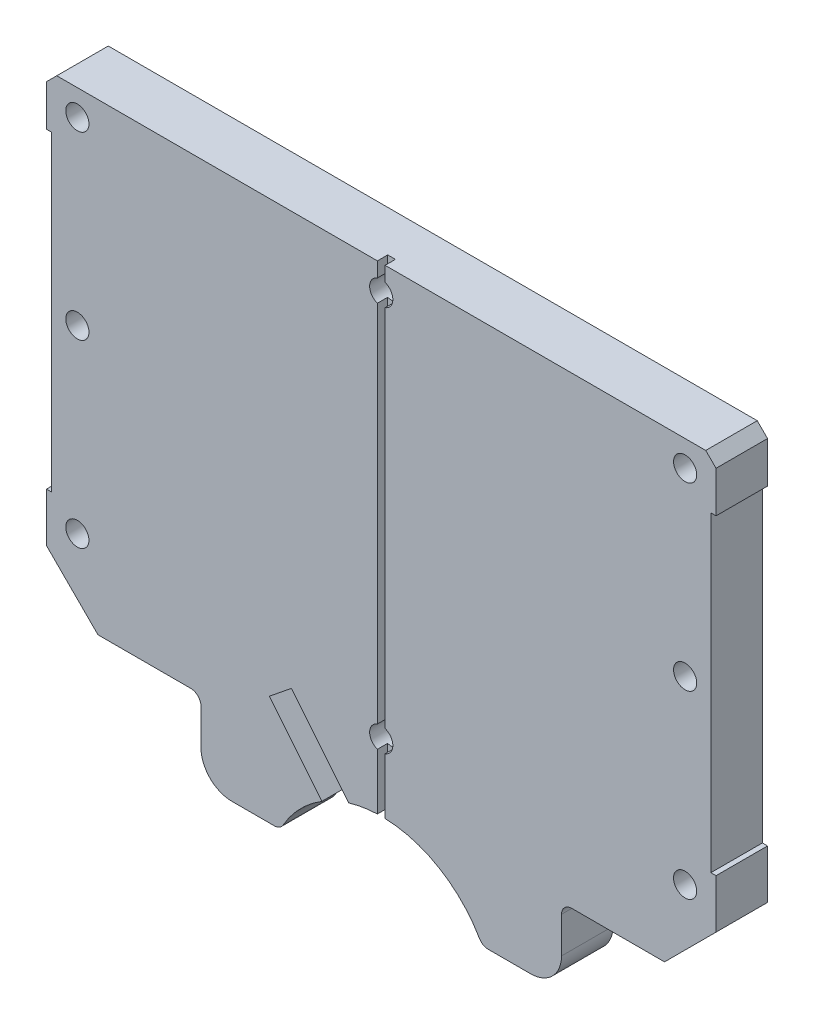
from build123d import *

# Parameters (mm, degrees)
SKETCH1_W                                            = 130
SKETCH1_H                                            = 105
BOSS_EXTRUDE1_DEPTH                                  = 5
SKETCH3_R                                            = 22
CUT_EXTRUDE2_DEPTH                                   = 85.150163399
SKETCH7_W                                            = 30
SKETCH7_H                                            = 10
CUT_EXTRUDE5_DEPTH                                   = 15
FILLET1_R                                            = 6
CHAMFER1_SIZE                                        = 10
FILLET2_R                                            = 2
CUT_EXTRUDE8_DEPTH                                   = 85.150163399
FILLET3_R                                            = 2
CHAMFER2_SIZE                                        = 2
SKETCH15_W                                           = 1
SKETCH15_H                                           = 60.5
CUT_EXTRUDE10_DEPTH                                  = 85.150163399
HOLE_SIZE_PER_SOCKET_HEAD_CAP_SCREW_TYPE_D           = 4.5
HOLE_SIZE_PER_SOCKET_HEAD_CAP_SCREW_TYPE_CBORE_D     = 8
HOLE_SIZE_PER_SOCKET_HEAD_CAP_SCREW_TYPE_CBORE_DEPTH = 4.5
M3_TAPPED_HOLE1_D                                    = 2.5
M3_TAPPED_HOLE1_DEPTH                                = 8.5
M3_TAPPED_HOLE1_TIP                                  = 0.751075774
SKETCH20_W                                           = 1.5
SKETCH20_H                                           = 105
CUT_EXTRUDE11_DEPTH                                  = 2


with BuildPart() as part:
    # Sketch1 → Boss-Extrude1 (new, symmetric)
    with BuildSketch(Plane.XY):
        Rectangle(SKETCH1_W, SKETCH1_H)
    extrude(amount=BOSS_EXTRUDE1_DEPTH, both=True)

    # Sketch3 → Cut-Extrude2 (cut, through all)
    with BuildSketch(Plane.XY.offset(5)):
        with Locations((0, -62.5)):
            Circle(SKETCH3_R)
    extrude(amount=-CUT_EXTRUDE2_DEPTH, mode=Mode.SUBTRACT)

    # Sketch7 → Cut-Extrude5 (cut)
    with BuildSketch(Plane.XZ.offset(52.5)):
        with Locations((-50, 0)):
            Rectangle(SKETCH7_W, SKETCH7_H)
        with Locations((50, 0)):
            Rectangle(SKETCH7_W, SKETCH7_H)
    extrude(amount=-CUT_EXTRUDE5_DEPTH, mode=Mode.SUBTRACT)

    # Fillet1
    fillet1_edges = [part.edges().sort_by_distance(p)[0] for p in [
        (-35, -52.5, 0),
        (35, -52.5, 0),
    ]]
    fillet(fillet1_edges, radius=FILLET1_R)

    # Chamfer1
    chamfer1_edges = [part.edges().sort_by_distance(p)[0] for p in [
        (-65, -37.5, 0),
        (65, -37.5, 0),
    ]]
    chamfer(chamfer1_edges, length=CHAMFER1_SIZE)

    # Fillet2
    fillet2_edges = [part.edges().sort_by_distance(p)[0] for p in [
        (-35, -37.5, 0),
        (35, -37.5, 0),
    ]]
    fillet(fillet2_edges, radius=FILLET2_R)

    # Sketch10 → Cut-Extrude8 (cut, through all)
    with BuildSketch(Plane.XY.offset(5)):
        Polygon((-21.710710609, -31.184123297), (-17.436407821, -27.722861146), (-4.85, -43.265780375), (-9.124302788, -46.727042526), align=None)
    extrude(amount=-CUT_EXTRUDE8_DEPTH, mode=Mode.SUBTRACT)

    # Fillet3
    fillet3_edges = [part.edges().sort_by_distance(p)[0] for p in [
        (-19.595917942, -52.5, 0),
        (19.595917942, -52.5, 0),
    ]]
    fillet(fillet3_edges, radius=FILLET3_R)

    # Chamfer2
    chamfer2_edges = [part.edges().sort_by_distance(p)[0] for p in [
        (-65, 52.5, 0),
        (65, 52.5, 0),
    ]]
    chamfer(chamfer2_edges, length=CHAMFER2_SIZE)

    # Sketch15 → Cut-Extrude10 (cut, through all)
    with BuildSketch(Plane(origin=(0, 0, -5), x_dir=(-1, 0, 0), z_dir=(0, 0, -1))):
        with Locations((-64.5, 12.25)):
            Rectangle(SKETCH15_W, SKETCH15_H)
        with Locations((64.5, 12.25)):
            Rectangle(SKETCH15_W, SKETCH15_H)
    extrude(amount=-CUT_EXTRUDE10_DEPTH, mode=Mode.SUBTRACT)

    # Hole size per socket head cap screw type 0 (through all)
    with Locations(Plane(origin=(-18.523886338, 13.049633662, -5), x_dir=(1, 0, 0), z_dir=(0, 0, -1))):
        with Locations((77.523886338, -34.450366338), (18.523886338, -34.450366338), (-40.476113662, -34.450366338), (-40.476113662, 0.549633662), (-40.476113662, 35.549633662), (18.523886338, 40.549633662), (77.523886338, 35.549633662), (77.523886338, 0.549633662)):
            CounterBoreHole(HOLE_SIZE_PER_SOCKET_HEAD_CAP_SCREW_TYPE_D / 2, HOLE_SIZE_PER_SOCKET_HEAD_CAP_SCREW_TYPE_CBORE_D / 2, HOLE_SIZE_PER_SOCKET_HEAD_CAP_SCREW_TYPE_CBORE_DEPTH)

    # M3 Tapped Hole1
    with Locations(Plane(origin=(-15.568631127, 3.135719595, -5), x_dir=(1, 0, 0), z_dir=(0, 0, -1))):
        with Locations((-7.431368873, 28.635719595)):
            Hole(M3_TAPPED_HOLE1_D / 2, depth=M3_TAPPED_HOLE1_DEPTH)
            with Locations((0, 0, -(M3_TAPPED_HOLE1_DEPTH + M3_TAPPED_HOLE1_TIP / 2))):  # 118° drill point
                Cone(0, M3_TAPPED_HOLE1_D / 2, M3_TAPPED_HOLE1_TIP, mode=Mode.SUBTRACT)

    # Sketch20 → Cut-Extrude11 (cut)
    with BuildSketch(Plane.XY.offset(5)):
        Rectangle(SKETCH20_W, SKETCH20_H)
    extrude(amount=-CUT_EXTRUDE11_DEPTH, mode=Mode.SUBTRACT)


solid = part.part
